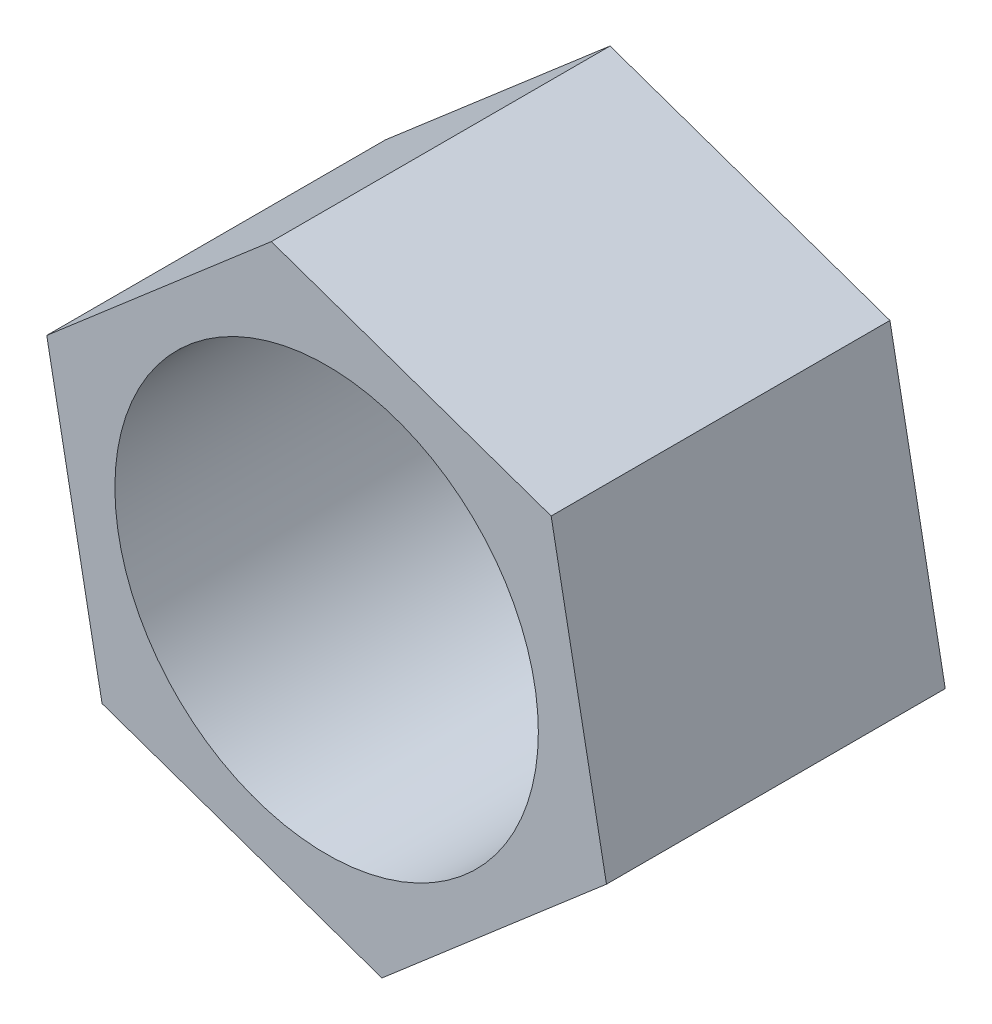
from build123d import *

# Parameters (mm, degrees)
SKETCH1_R           = 6.35
BOSS_EXTRUDE1_DEPTH = 10.16
SCALE1_SCALE        = 2


with BuildPart() as part:
    # Sketch1 → Boss-Extrude1 (new body)
    with BuildSketch(Plane.XY):
        Polygon((6.73459618, 5.803215857), (-1.658434266, 8.733939305), (-8.393030446, 2.930723448), (-6.73459618, -5.803215857), (1.658434266, -8.733939305), (8.393030446, -2.930723448), align=None)
        Circle(SKETCH1_R, mode=Mode.SUBTRACT)
    extrude(amount=BOSS_EXTRUDE1_DEPTH)


with BuildPart() as part_1:
    # Scale1: scaled about (0, 0, 0)
    add(part.part.scale(SCALE1_SCALE))


solid = part_1.part
